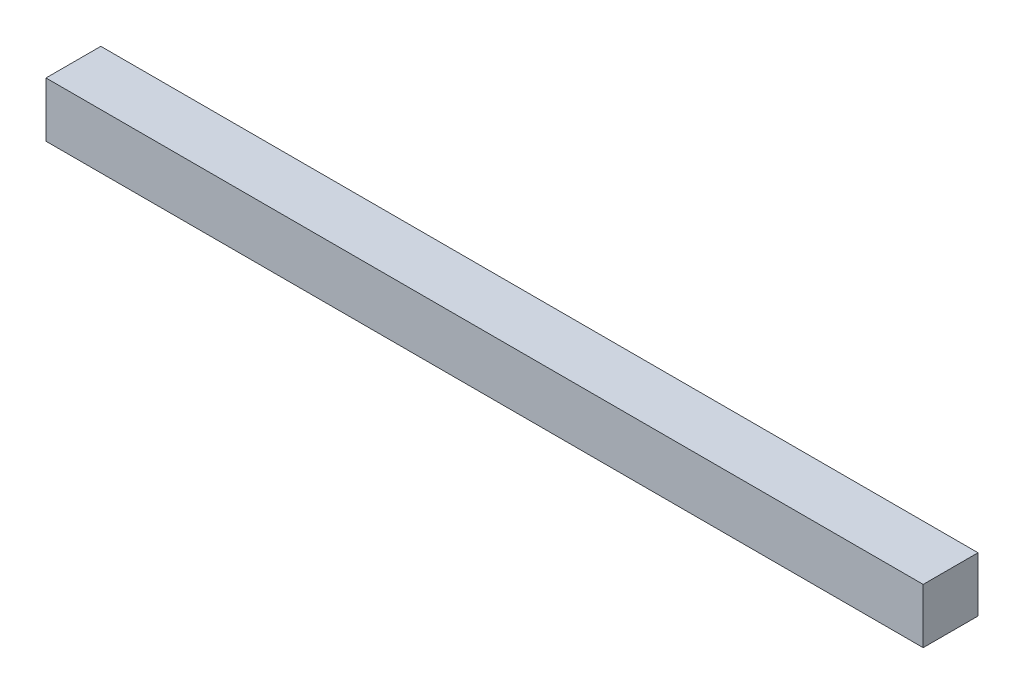
from build123d import *

# Parameters (mm, degrees)
SKETCH_1_W      = 80
SKETCH_1_H      = 5
EXTRUDE_1_DEPTH = 5


with BuildPart() as part:
    # 草图1 → 凸台-拉伸1 (new body)
    with BuildSketch(Plane.XY):
        with Locations((40, 2.5)):
            Rectangle(SKETCH_1_W, SKETCH_1_H)
    extrude(amount=EXTRUDE_1_DEPTH)


solid = part.part
